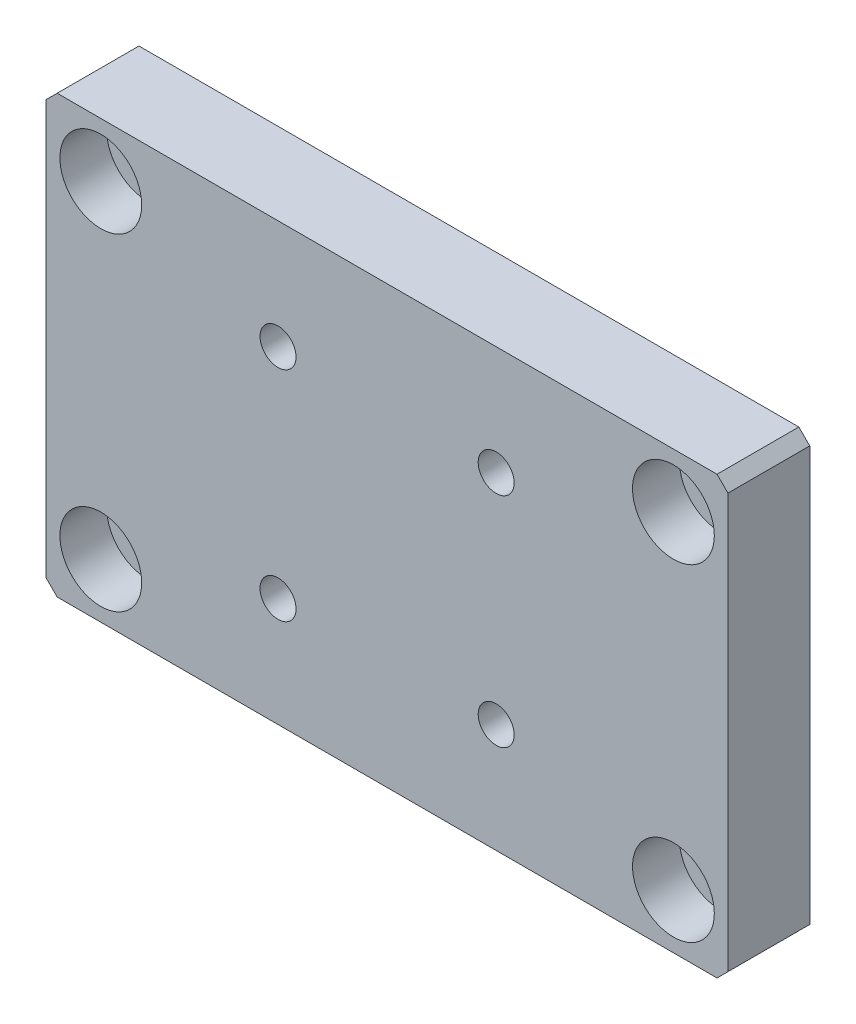
SolidWorks part; units mm, degrees
ref_plane "前视基准面" through (0, 0, 0) normal (0, 0, 1) x (1, 0, 0)
ref_plane "上视基准面" through (0, 0, 0) normal (0, 1, 0) x (1, 0, 0)
ref_plane "右视基准面" through (0, 0, 0) normal (1, 0, 0) x (0, 0, -1)
sketch "草图1" plane through (0, 0, 0) normal (0, 0, 1) x (1, 0, 0)
  line L1 (-62.5, 40) -> (62.5, 40)
  line L2 (-62.5, 40) -> (-62.5, -40)
  line L3 (-62.5, -40) -> (62.5, -40)
  line L4 (62.5, 40) -> (62.5, -40)
  line L5 (-62.5, 40) -> (62.5, -40) construction
  line L6 (-62.5, -40) -> (62.5, 40) construction
  point P0 (0, 0)
  dimension "D1" = 125
  dimension "D2" = 80
extrude "凸台-拉伸1" add sketch "草图1" along normal mid plane 15
hole_wizard "M8 六角凹头螺钉的柱形沉头孔1" positions "草图3" profile "草图2" counterbore size "M8" standard "ISO" end condition through all
sketch "草图3" plane through (0, 0, 7.5) normal (0, 0, 1) x (1, 0, 0)
  line L0 (0, 0) -> (0, 24.7948) construction
  point P0 (-52.5, 30)
  point P2 (-52.5, -30)
  point P21 (52.5, -30)
  point P22 (52.5, 30)
  dimension "D1" = 52.5
  dimension "D2" = 60
  dimension "D3" = 30
sketch "草图2" plane through (-52.5, 30, 7.5) normal (1, 0, 0) x (0, -1, 0)
  line L0 (0, 0) -> (0, 15)
  line L1 (0, 15) -> (4.5, 15)
  line L3 (4.5, 15) -> (4.5, 8.6)
  line L4 (4.5, 8.6) -> (7.5, 8.6)
  line L5 (7.5, 8.6) -> (7.5, 0)
  line L7 (7.5, 0) -> (0, 0)
  line L11 (0, -6.35) -> (0, 107.95) construction
  dimension "通孔孔直径" = 9
  dimension "通孔孔深度" = 15
  dimension "柱形沉头孔直径" = 15
  dimension "柱形沉头孔深度" = 8.6
hole_wizard "M6 六角凹头螺钉的柱形沉头孔1" positions "草图5" profile "草图4" counterbore size "M6" standard "ISO" end condition through all
sketch "草图5" plane through (0, 0, -7.5) normal (0, 0, -1) x (-1, 0, 0)
  line L0 (0, 0) -> (0, 24.7948) construction
  point P0 (-20, -20)
  point P2 (-20, 20)
  point P15 (20, -20)
  point P16 (20, 20)
  dimension "D1" = 40
  dimension "D2" = 20
  dimension "D3" = 20
sketch "草图4" plane through (20, -20, -7.5) normal (1, 0, 0) x (0, 1, 0)
  line L0 (0, 0) -> (0, 15)
  line L1 (0, 15) -> (3.3, 15)
  line L3 (3.3, 15) -> (3.3, 6.4)
  line L4 (3.3, 6.4) -> (5.5, 6.4)
  line L5 (5.5, 6.4) -> (5.5, 0)
  line L7 (5.5, 0) -> (0, 0)
  line L11 (0, -6.35) -> (0, 107.95) construction
  dimension "通孔孔直径" = 6.6
  dimension "通孔孔深度" = 15
  dimension "柱形沉头孔直径" = 11
  dimension "柱形沉头孔深度" = 6.4
chamfer "倒角1" distance 2 angle 45 4 edges at (62.5, 40, 0) (62.5, -40, 0) (-62.5, -40, 0) (-62.5, 40, 0)
